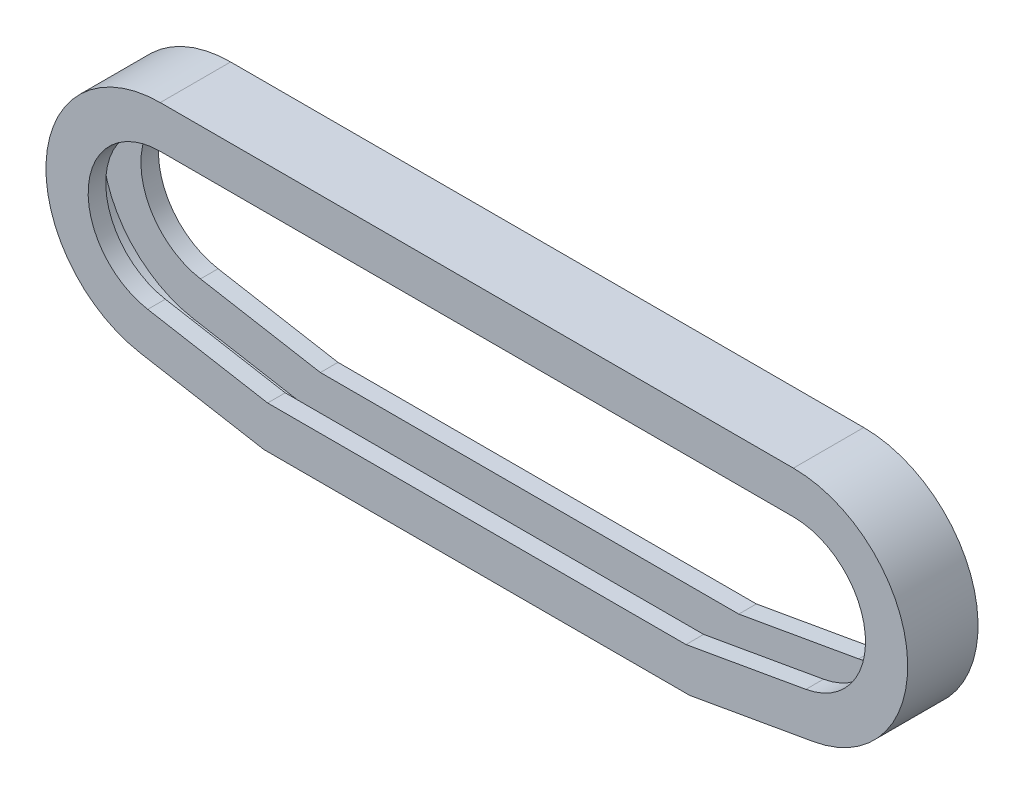
from build123d import *

# Parameters (mm, degrees)
BOSS_EXTRUDE1_DEPTH = 10
CUT_EXTRUDE1_DEPTH  = 5


with BuildPart() as part:
    # Sketch2 → Boss-Extrude1 (new, symmetric)
    with BuildSketch(Plane.XY):
        with BuildLine():
            Line((-90, 32.5), (90, 32.5))
            ThreePointArc((90, 32.5), (122.376327688, 2.832561639), (95.643565774, -32.006251973))
            Line((95.643565774, -32.006251973), (60.524931981, -38.198614636))
            Line((60.524931981, -38.198614636), (-60.524931981, -38.198614636))
            Line((-60.524931981, -38.198614636), (-95.643565774, -32.006251973))
            ThreePointArc((-95.643565774, -32.006251973), (-122.376327688, 2.832561639), (-90, 32.5))
        make_face()
        with BuildLine():
            Line((-90, 20.5), (90, 20.5))
            ThreePointArc((90, 20.5), (110.421991311, 1.786692726), (93.559787642, -20.188558937))
            Line((93.559787642, -20.188558937), (59.475068019, -26.198614636))
            Line((59.475068019, -26.198614636), (-59.475068019, -26.198614636))
            Line((-59.475068019, -26.198614636), (-93.559787642, -20.188558937))
            ThreePointArc((-93.559787642, -20.188558937), (-110.421991311, 1.786692726), (-90, 20.5))
        make_face(mode=Mode.SUBTRACT)
    extrude(amount=BOSS_EXTRUDE1_DEPTH, both=True)

    # Sketch8 → Cut-Extrude1 (cut, symmetric)
    with BuildSketch(Plane.XY):
        with BuildLine():
            Line((60.437443318, -37.198614636), (95.469917597, -31.02144422))
            ThreePointArc((95.469917597, -31.02144422), (121.38013299, 2.745405897), (90, 31.5))
            Line((90, 31.5), (-90, 31.5))
            ThreePointArc((-90, 31.5), (-121.38013299, 2.745405897), (-95.469917597, -31.02144422))
            Line((-95.469917597, -31.02144422), (-60.437443318, -37.198614636))
            Line((-60.437443318, -37.198614636), (60.437443318, -37.198614636))
        make_face()
    extrude(amount=CUT_EXTRUDE1_DEPTH, both=True, mode=Mode.SUBTRACT)


solid = part.part
